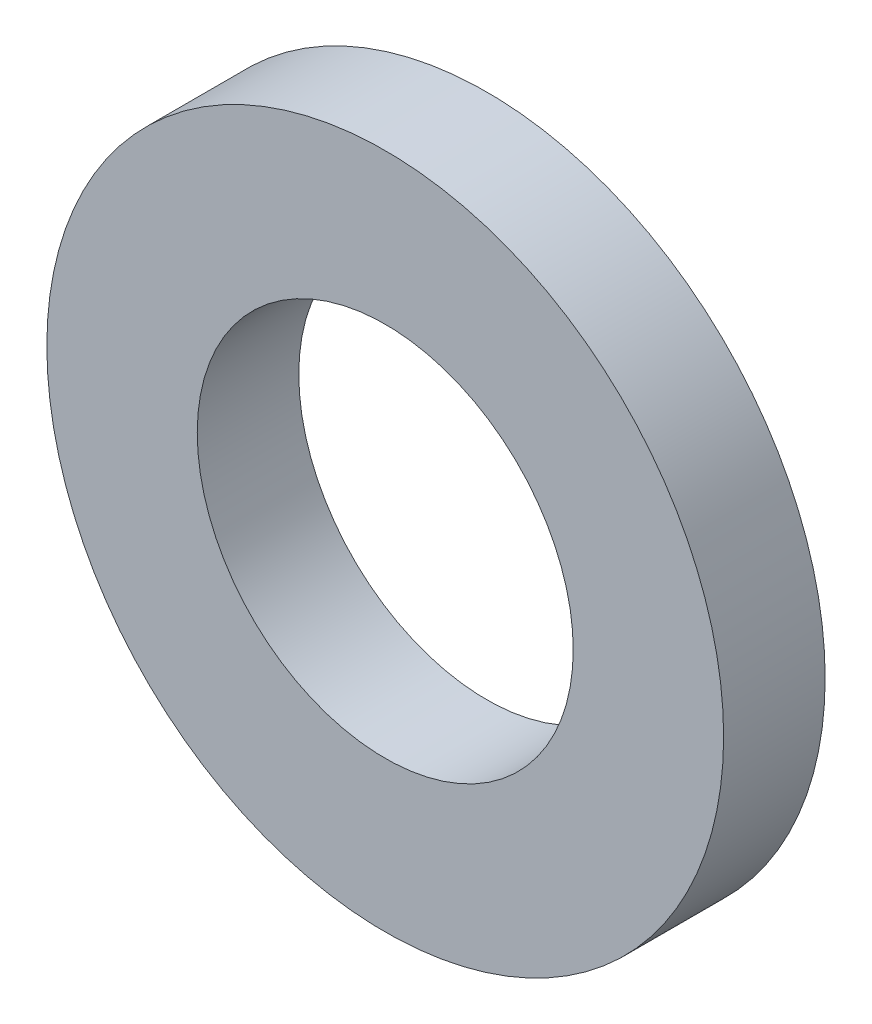
SolidWorks part; units mm, degrees
material "合金钢"
ref_plane "Front Plane" through (0, 0, 0) normal (0, 0, 1) x (1, 0, 0)
ref_plane "Top Plane" through (0, 0, 0) normal (0, 1, 0) x (1, 0, 0)
ref_plane "Right Plane" through (0, 0, 0) normal (1, 0, 0) x (0, 0, -1)
sketch "Sketch1" plane through (0, 0, 0) normal (0, 0, 1) x (1, 0, 0)
  circle A0 centre (0, 0) radius 9
  circle A1 centre (0, 0) radius 5
extrude "Boss-Extrude1" add sketch "Sketch1" along normal blind 2.7
